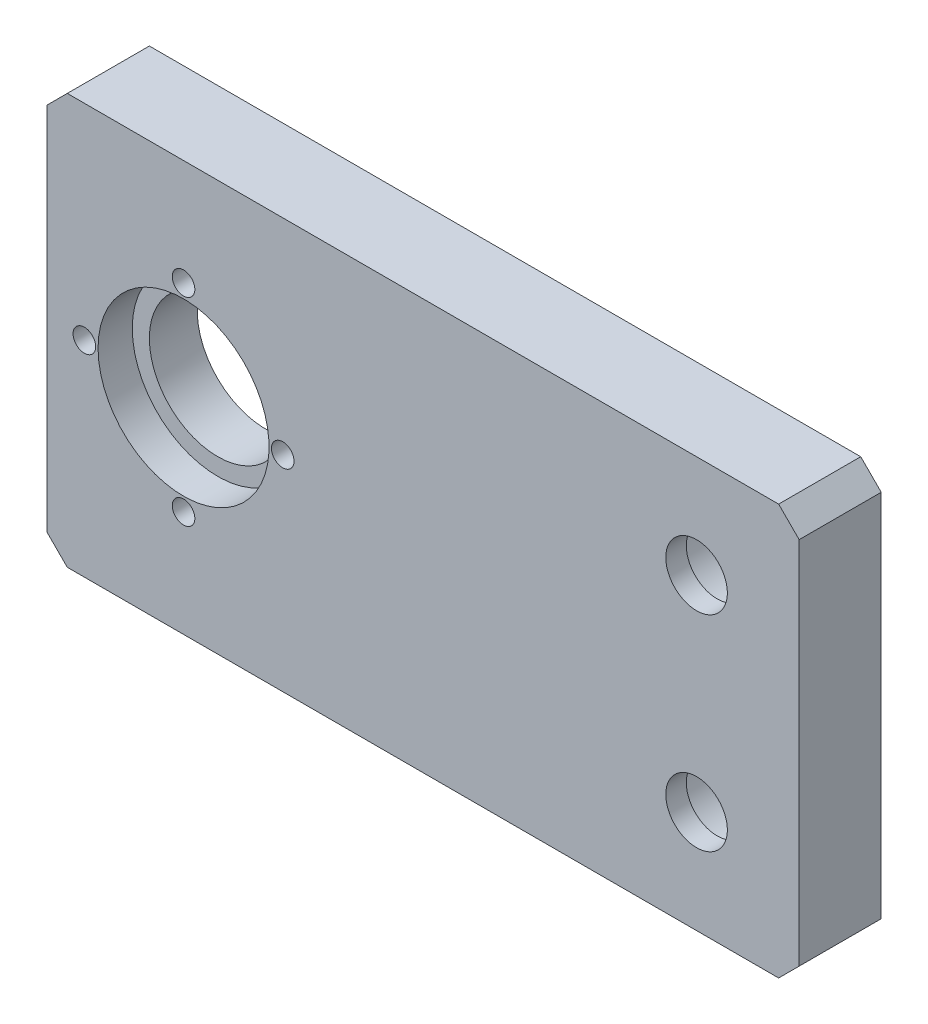
from build123d import *

# Parameters (mm, degrees)
SKETCH1_W                                            = 110
SKETCH1_H                                            = 60
BOSS_EXTRUDE1_DEPTH                                  = 12
SKETCH2_R                                            = 12.5
CUT_EXTRUDE1_DEPTH                                   = 5
SKETCH3_R                                            = 10
CUT_EXTRUDE3_DEPTH                                   = 64.788713735
CHAMFER1_SIZE                                        = 3
M4_TAPPED_HOLE1_D                                    = 3.3
CBORE_FOR_M8_HEXAGON_SOCKET_HEAD_CAP_SCR_D           = 9
CBORE_FOR_M8_HEXAGON_SOCKET_HEAD_CAP_SCR_CBORE_D     = 15
CBORE_FOR_M8_HEXAGON_SOCKET_HEAD_CAP_SCR_CBORE_DEPTH = 9


with BuildPart() as part:
    # Sketch1 → Boss-Extrude1 (new body)
    with BuildSketch(Plane.XY):
        Rectangle(SKETCH1_W, SKETCH1_H)
    extrude(amount=BOSS_EXTRUDE1_DEPTH)

    # Sketch2 → Cut-Extrude1 (cut)
    with BuildSketch(Plane(origin=(0, 0, 12), x_dir=(-1, 0, 0), z_dir=(0, 0, -1))):
        with Locations((35, 0)):
            Circle(SKETCH2_R)
    extrude(amount=CUT_EXTRUDE1_DEPTH, mode=Mode.SUBTRACT)

    # Sketch3 → Cut-Extrude3 (cut, through all)
    with BuildSketch(Plane.XY.offset(12)):
        with Locations((-35, 0)):
            Circle(SKETCH3_R)
    extrude(amount=-CUT_EXTRUDE3_DEPTH, mode=Mode.SUBTRACT)

    # Chamfer1
    chamfer1_edges = [part.edges().sort_by_distance(p)[0] for p in [
        (55, -30, 6),
        (-55, -30, 6),
        (-55, 30, 6),
        (55, 30, 6),
    ]]
    chamfer(chamfer1_edges, length=CHAMFER1_SIZE)

    # M4 Tapped Hole1 (through all)
    with Locations(Plane.XY.offset(12)):
        with Locations((-35, 14.5), (-20.5, 0), (-49.5, 0), (-35, -14.5)):
            Hole(M4_TAPPED_HOLE1_D / 2)

    # CBORE for M8 Hexagon socket head cap screws1 (through all)
    with Locations(Plane(origin=(0, 0, 0), x_dir=(-1, 0, 0), z_dir=(0, 0, -1))):
        with Locations((-40, 15), (-40, -15)):
            CounterBoreHole(CBORE_FOR_M8_HEXAGON_SOCKET_HEAD_CAP_SCR_D / 2, CBORE_FOR_M8_HEXAGON_SOCKET_HEAD_CAP_SCR_CBORE_D / 2, CBORE_FOR_M8_HEXAGON_SOCKET_HEAD_CAP_SCR_CBORE_DEPTH)


solid = part.part
